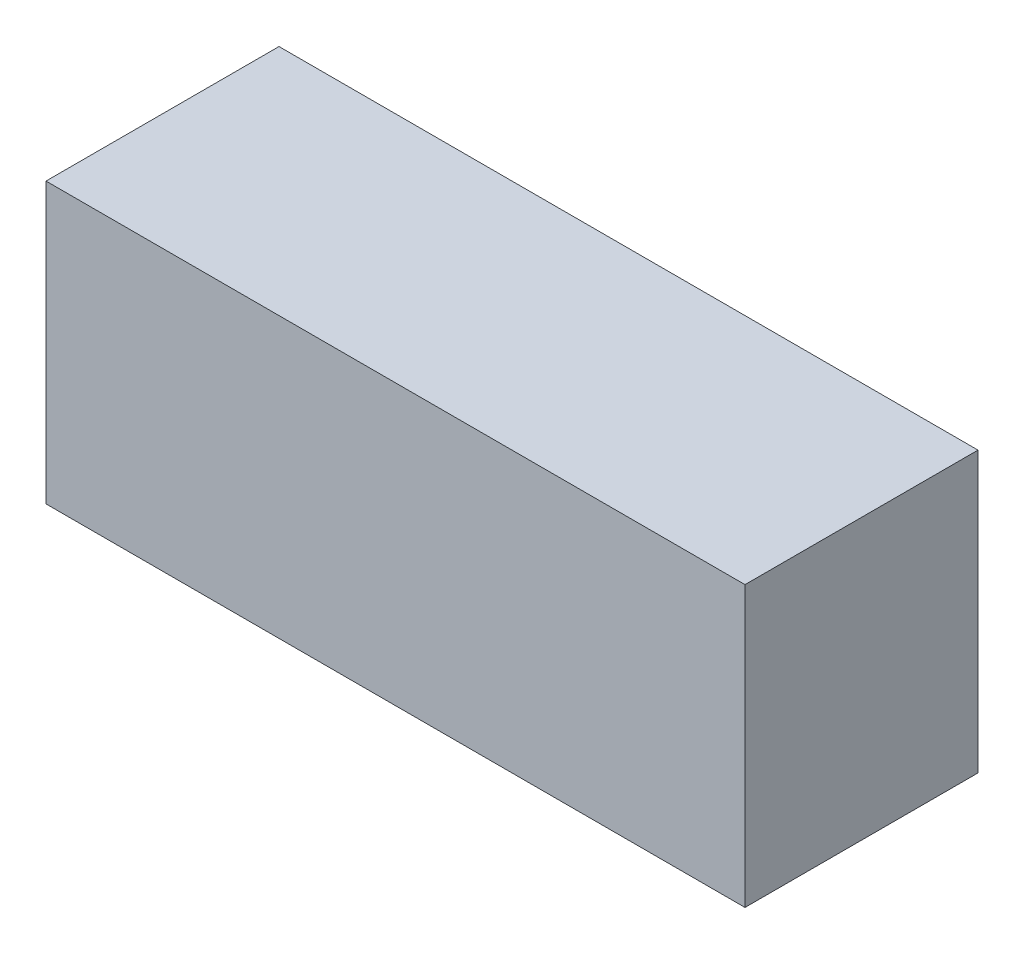
from build123d import *

# Parameters (mm, degrees)
SKETCH_1_W      = 30
SKETCH_1_H      = 12
EXTRUDE_1_DEPTH = 5


with BuildPart() as part:
    # 草图1 → 凸台-拉伸1 (new, symmetric)
    with BuildSketch(Plane.XY):
        Rectangle(SKETCH_1_W, SKETCH_1_H)
    extrude(amount=EXTRUDE_1_DEPTH, both=True)


solid = part.part
